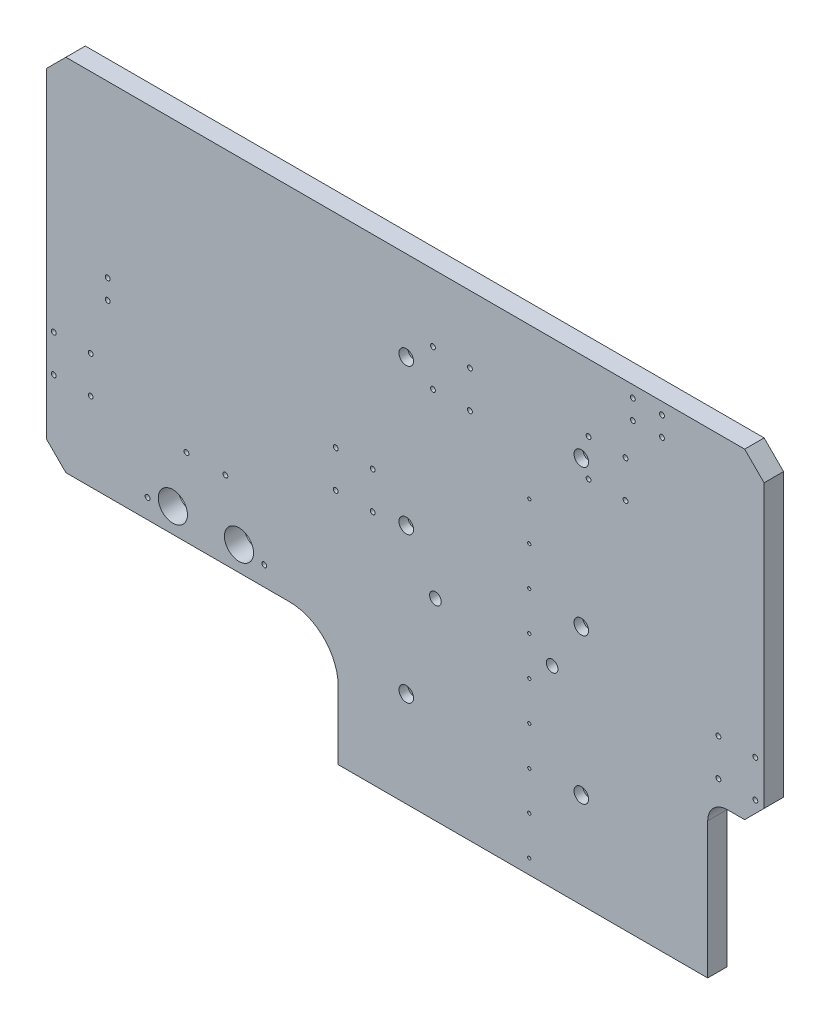
from build123d import *

# Parameters (mm, degrees)
BOSS_EXTRUDE3_DEPTH                                  = 20
CHAMFER1_SIZE                                        = 20
CUT_EXTRUDE3_DEPTH                                   = 697.867993238
SKETCH6_W                                            = 62
SKETCH6_H                                            = 330
CUT_EXTRUDE4_DEPTH                                   = 697.867993238
CHAMFER3_SIZE                                        = 20
M6_TAPPED_HOLE1_D                                    = 5
M4_TAPPED_HOLE1_D                                    = 3.3
M6_TAPPED_HOLE2_D                                    = 5
SKETCH17_R                                           = 15
CUT_EXTRUDE5_DEPTH                                   = 645.83443917
HOLE_SIZE_PER_SOCKET_HEAD_CAP_SCREW_TYPE_D           = 9
HOLE_SIZE_PER_SOCKET_HEAD_CAP_SCREW_TYPE_CBORE_D     = 15
HOLE_SIZE_PER_SOCKET_HEAD_CAP_SCREW_TYPE_CBORE_DEPTH = 9
SKETCH20_R                                           = 6
CUT_EXTRUDE6_DEPTH                                   = 645.83443917
M6_TAPPED_HOLE3_D                                    = 5
M6_TAPPED_HOLE4_D                                    = 5


with BuildPart() as part:
    # Sketch2 → Boss-Extrude3 (new body)
    with BuildSketch(Plane.XY):
        with BuildLine():
            Line((-205.987531774, -243.832636788), (44.012468226, -243.832636788))
            ThreePointArc((44.012468226, -243.832636788), (79.367807285, -258.477297729), (94.012468226, -293.832636788))
            Line((94.012468226, -293.832636788), (94.012468226, -363.832636788))
            Line((94.012468226, -363.832636788), (594.012468226, -363.832636788))
            Line((594.012468226, -363.832636788), (594.012468226, 126.167363212))
            Line((594.012468226, 126.167363212), (-205.987531774, 126.167363212))
            Line((-205.987531774, 126.167363212), (-205.987531774, -243.832636788))
        make_face()
    extrude(amount=BOSS_EXTRUDE3_DEPTH)

    # Chamfer1
    chamfer1_edges = [part.edges().sort_by_distance(p)[0] for p in [
        (-205.987531774, -243.832636788, 10),
        (-205.987531774, 126.167363212, 10),
        (594.012468226, 126.167363212, 10),
    ]]
    chamfer(chamfer1_edges, length=CHAMFER1_SIZE)

    # Sketch5 → Cut-Extrude3 (cut, through all)
    with BuildSketch(Plane.XY.offset(20)):
        with BuildLine():
            Line((594.012468226, -363.832636788), (474.012468226, -363.832636788))
            Line((474.012468226, -363.832636788), (474.012468226, -223.832636788))
            ThreePointArc((474.012468226, -223.832636788), (479.870332602, -209.690501165), (494.012468226, -203.832636788))
            Line((494.012468226, -203.832636788), (594.012468226, -203.832636788))
            Line((594.012468226, -203.832636788), (594.012468226, -363.832636788))
        make_face()
    extrude(amount=-CUT_EXTRUDE3_DEPTH, mode=Mode.SUBTRACT)

    # Sketch6 → Cut-Extrude4 (cut, through all)
    with BuildSketch(Plane.XY.offset(20)):
        with Locations((563.012468226, -38.832636788)):
            Rectangle(SKETCH6_W, SKETCH6_H)
    extrude(amount=-CUT_EXTRUDE4_DEPTH, mode=Mode.SUBTRACT)

    # Chamfer3
    chamfer3_edges = [part.edges().sort_by_distance(p)[0] for p in [
        (532.012468226, -203.832636788, 10),
        (532.012468226, 126.167363212, 10),
    ]]
    chamfer(chamfer3_edges, length=CHAMFER3_SIZE)

    # M6 Tapped Hole1 (through all)
    with Locations(Plane.XY.offset(20)):
        with Locations((427.012468226, 114.167363212), (397.012468226, 114.167363212), (397.012468226, 94.167363212), (427.012468226, 94.167363212)):
            Hole(M6_TAPPED_HOLE1_D / 2)

    # M4 Tapped Hole1 (through all)
    with Locations(Plane.XY.offset(20)):
        with Locations((290.512468226, -348.832636788), (290.512468226, -308.832636788), (290.512468226, -268.832636788), (290.512468226, -228.832636788), (290.512468226, -188.832636788), (290.512468226, -148.832636788), (290.512468226, -108.832636788), (290.512468226, -68.832636788), (290.512468226, -28.832636788)):
            Hole(M4_TAPPED_HOLE1_D / 2)

    # M6 Tapped Hole2 (through all)
    with Locations(Plane.XY.offset(20)):
        with Locations((-61.987531774, -163.832636788), (-101.987531774, -223.832636788), (18.012468226, -223.832636788), (-21.987531774, -163.832636788)):
            Hole(M6_TAPPED_HOLE2_D / 2)

    # Sketch17 → Cut-Extrude5 (cut, through all)
    with BuildSketch(Plane.XY.offset(20)):
        with Locations((-75.987531774, -218.832636788)):
            Circle(SKETCH17_R)
        with Locations((-7.987531774, -218.832636788)):
            Circle(SKETCH17_R)
    extrude(amount=-CUT_EXTRUDE5_DEPTH, mode=Mode.SUBTRACT)

    # Hole size per socket head cap screw type 1 (through all)
    with Locations(Plane.XY.offset(20)):
        with Locations((164.012468226, 34.167363212), (344.012468226, 34.167363212), (344.012468226, -115.832636788), (164.012468226, -115.832636788), (164.012468226, -265.832636788), (344.012468226, -265.832636788)):
            CounterBoreHole(HOLE_SIZE_PER_SOCKET_HEAD_CAP_SCREW_TYPE_D / 2, HOLE_SIZE_PER_SOCKET_HEAD_CAP_SCREW_TYPE_CBORE_D / 2, HOLE_SIZE_PER_SOCKET_HEAD_CAP_SCREW_TYPE_CBORE_DEPTH)

    # Sketch20 → Cut-Extrude6 (cut, through all)
    with BuildSketch(Plane.XY.offset(20)):
        with Locations((194.012468226, -165.832636788)):
            Circle(SKETCH20_R)
        with Locations((314.012468226, -165.832636788)):
            Circle(SKETCH20_R)
    extrude(amount=-CUT_EXTRUDE6_DEPTH, mode=Mode.SUBTRACT)

    # M6 Tapped Hole3 (through all)
    with Locations(Plane.XY.offset(20)):
        with Locations((-198.487531774, -124.832636788), (-160.487531774, -124.832636788), (-160.487531774, -162.832636788), (-198.487531774, -162.832636788), (191.512468226, 19.167363212), (229.512468226, 19.167363212), (229.512468226, 57.167363212), (191.512468226, 57.167363212), (389.512468226, 19.167363212), (351.512468226, 19.167363212), (389.512468226, 57.167363212), (351.512468226, 57.167363212), (523.012468226, -142.832636788), (485.012468226, -142.832636788), (485.012468226, -180.832636788), (523.012468226, -180.832636788), (91.512468226, -82.832636788), (129.512468226, -82.832636788), (129.512468226, -120.832636788), (91.512468226, -120.832636788)):
            Hole(M6_TAPPED_HOLE3_D / 2)

    # M6 Tapped Hole4 (through all)
    with Locations(Plane.XY.offset(20)):
        with Locations((-142.987531774, -48.832636788), (-142.987531774, -68.832636788)):
            Hole(M6_TAPPED_HOLE4_D / 2)


solid = part.part
